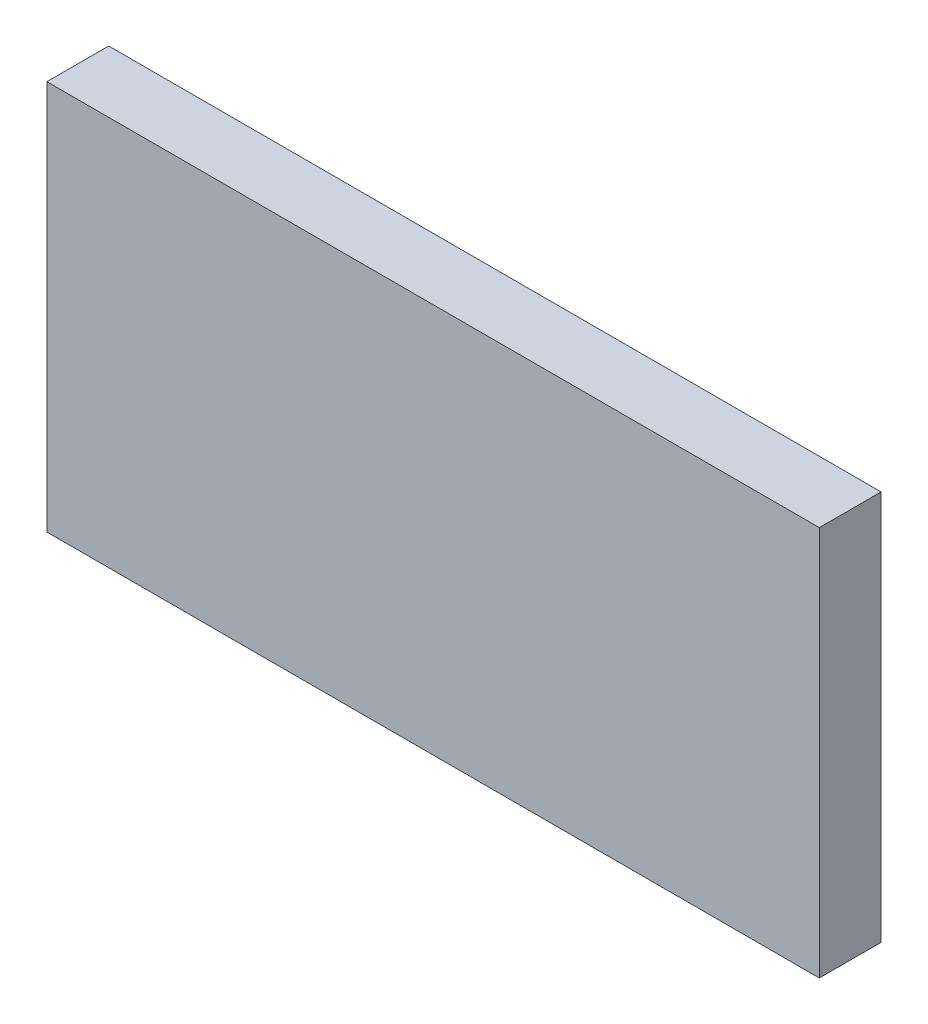
SolidWorks part; units mm, degrees
material "Q235B"
ref_plane "Front Plane" through (0, 0, 0) normal (0, 0, 1) x (1, 0, 0)
ref_plane "Top Plane" through (0, 0, 0) normal (0, 1, 0) x (1, 0, 0)
ref_plane "Right Plane" through (0, 0, 0) normal (1, 0, 0) x (0, 0, -1)
sketch "Sketch1" plane through (0, 0, 0) normal (0, 0, 1) x (1, 0, 0)
  line L1 (100, -50.5) -> (-100, -50.5)
  line L2 (100, -50.5) -> (100, 50.5)
  line L3 (100, 50.5) -> (-100, 50.5)
  line L4 (-100, -50.5) -> (-100, 50.5)
  line L5 (100, -50.5) -> (-100, 50.5) construction
  line L6 (100, 50.5) -> (-100, -50.5) construction
  point P0 (0, 0)
  dimension "D1" = 101
  dimension "D2" = 200
extrude "Boss-Extrude1" add sketch "Sketch1" along normal mid plane 16
